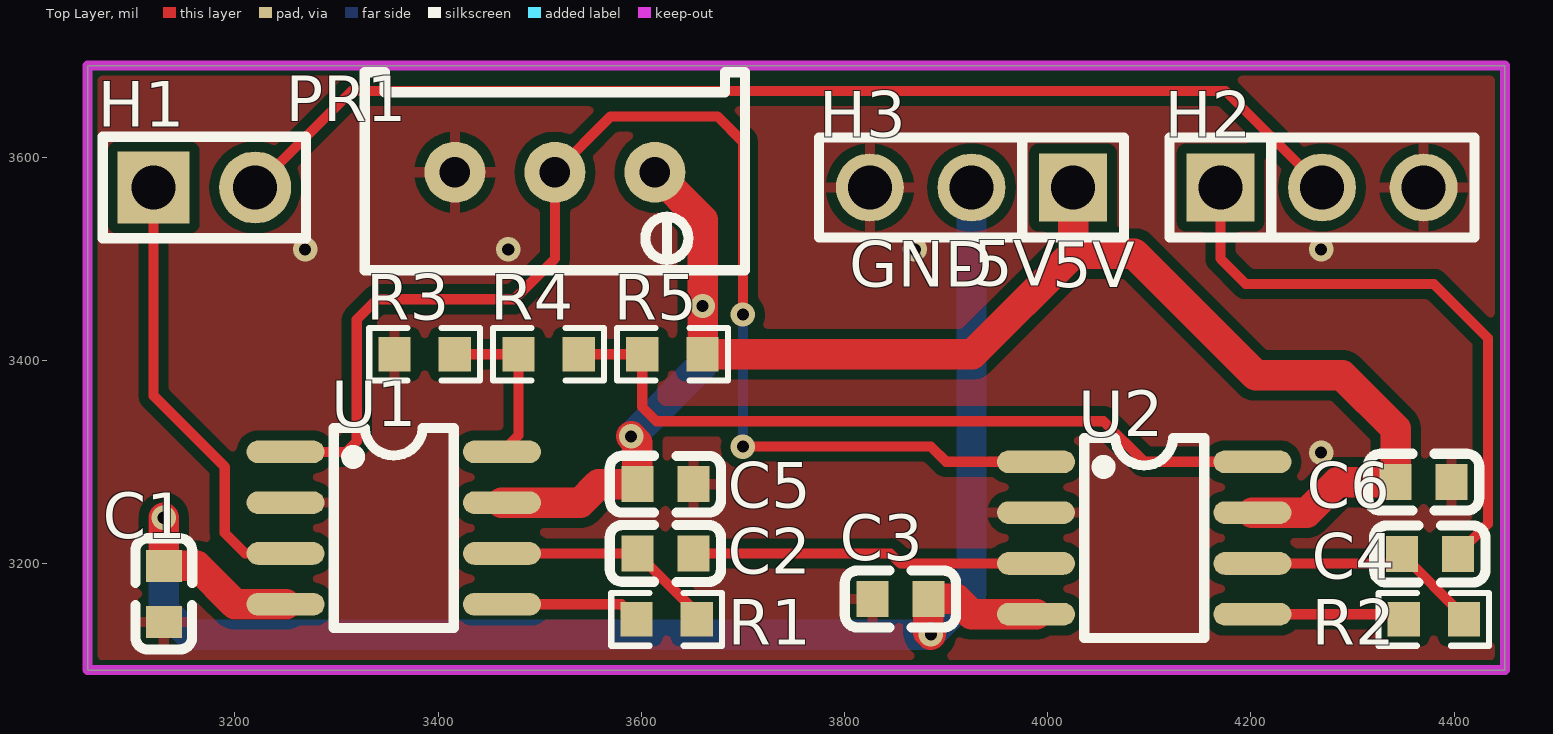
[diagram p0: Top Layer view]
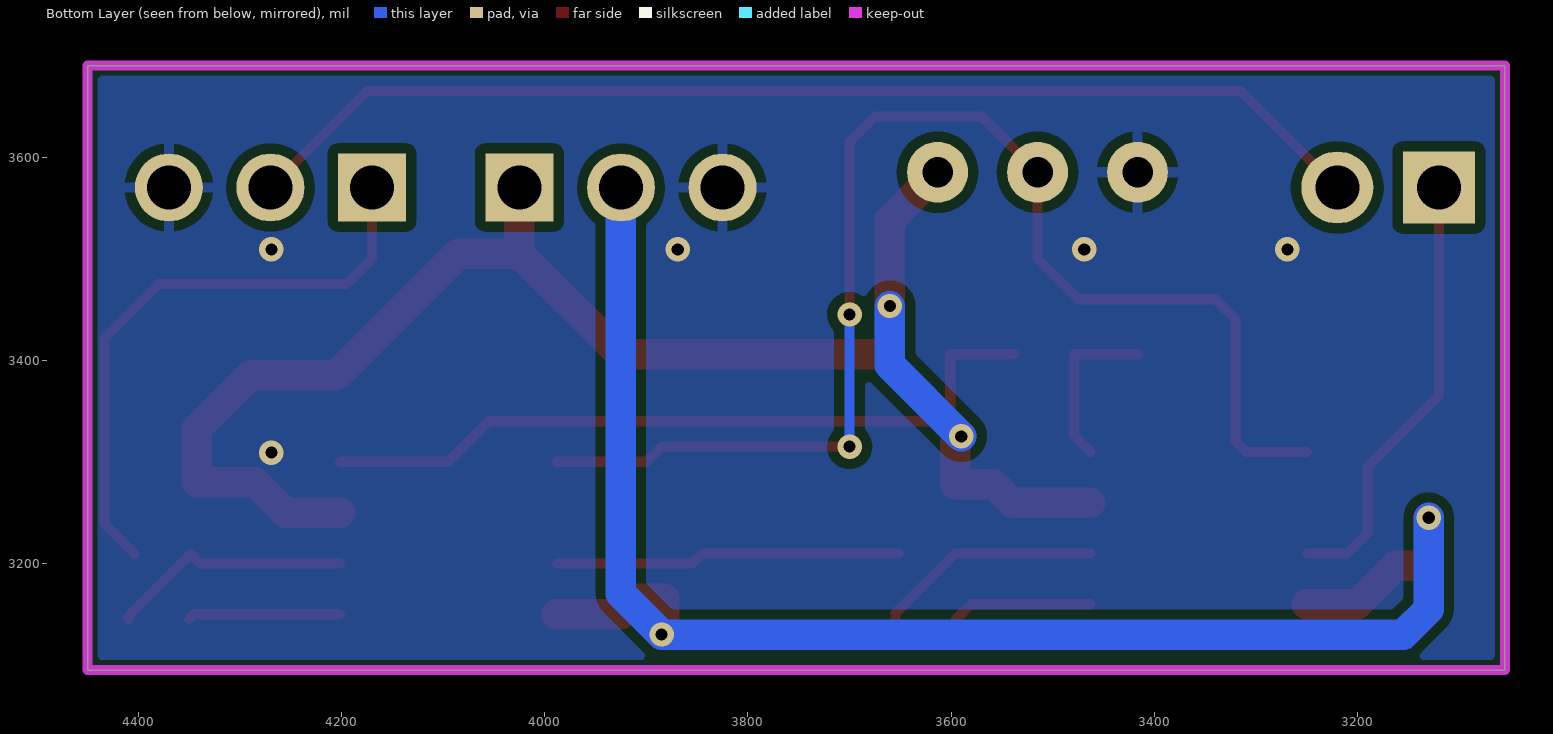
[diagram p1: Bottom Layer view, seen from below]
# Altium PCB MISC89042.pcbdoc
Units mil, origin at the board's own origin, x right, y up, seen from the top; angles counter-clockwise.
Board outline 1395 x 595 mil, 2 copper layers (Top Layer, Bottom Layer), stack 62.206 mil thick; 17 components, 14 nets, 49 pads, 11 vias.

## Layer stack, top to bottom
Top Solder Mask Layer: solder mask 0.394, Dk 3.3
Top Layer: signal copper 1.379
Dielectric1: surface 59.449, FR4, Dk 4.5
Bottom Layer: signal copper 1.378
Bottom Solder Mask Layer: solder mask 0.394, Dk 3.3

## Board outline
3055,3690 3055,3095 4450,3095 4450,3690

## Design rules (kind name [scope] priority, off if disabled: settings)
BoardOutlineClearance copperThickness2oz_1 [All] p2 off: genericclearance=7.99 ignorepadtopadclearanceinfootprint=FALSE except(0: Arc-SplitContinuation Track-SplitContinuation SMDPad-SplitContinuation THPad-SplitContinuation Via-SplitContinuation Fill-SplitContinuation Region-SplitContinuation Poly-SplitContinuation Text-SplitContinuation Hole-SplitContinuation; 5.98: Arc-CutoutEdge SMDPad-CutoutEdge THPad-CutoutEdge Via-CutoutEdge Fill-CutoutEdge Region-CutoutEdge Text-CutoutEdge; 6.93: Hole-OutlineEdge Hole-CutoutEdge; 10: Poly-OutlineEdge Poly-CutoutEdge; 11.81: Arc-OutlineEdge Track-OutlineEdge SMDPad-OutlineEdge THPad-OutlineEdge Via-OutlineEdge Fill-OutlineEdge Region-OutlineEdge Text-OutlineEdge Track-CutoutEdge)
BoardOutlineClearance copperThickness1oz_1 [All] p4: genericclearance=4.02 ignorepadtopadclearanceinfootprint=FALSE except(0: Arc-SplitContinuation Track-SplitContinuation SMDPad-SplitContinuation THPad-SplitContinuation Via-SplitContinuation Fill-SplitContinuation Region-SplitContinuation Poly-SplitContinuation Text-SplitContinuation Hole-SplitContinuation; 6: SMDPad-CutoutEdge THPad-CutoutEdge Via-CutoutEdge Fill-CutoutEdge Region-CutoutEdge Text-CutoutEdge; 6.93: Hole-OutlineEdge Hole-CutoutEdge; 10: Poly-OutlineEdge Poly-CutoutEdge; 11.8: Arc-OutlineEdge Track-OutlineEdge SMDPad-OutlineEdge THPad-OutlineEdge Via-OutlineEdge Fill-OutlineEdge Region-OutlineEdge Text-OutlineEdge; 11.81: Arc-CutoutEdge Track-CutoutEdge)
Clearance copperThickness2oz [All] p1 off: gap=7.99 ignorepadtopadclearanceinfootprint=FALSE except(5.98: SMDPad-Track SMDPad-SMDPad THPad-Track SMDPad-THPad THPad-THPad Track-Via SMDPad-Via THPad-Via Via-Via Fill-Track Region-Track Fill-SMDPad Region-SMDPad Fill-THPad Region-THPad Fill-Via Region-Via Fill-Fill Fill-Region Region-Region Arc-Track Arc-SMDPad Arc-THPad Arc-Via Fill-Arc Region-Arc Arc-Arc Text-Track SMDPad-Text Text-THPad Text-Via Fill-Text Region-Text Arc-Text Text-Text; 6.93: Hole-Track Hole-SMDPad Hole-THPad Hole-Via Fill-Hole Region-Hole Hole-Arc Hole-Text; 10: Poly-Track Poly-SMDPad Poly-THPad Poly-Via Poly-Fill Poly-Region Poly-Poly Poly-Arc Poly-Text Poly-Hole)
Clearance copperThickness1oz [All] p3: gap=4.02 ignorepadtopadclearanceinfootprint=FALSE except(5.98: SMDPad-Track SMDPad-SMDPad THPad-Track SMDPad-THPad THPad-THPad Track-Via SMDPad-Via THPad-Via Via-Via Fill-Track Region-Track Fill-SMDPad Region-SMDPad Fill-THPad Region-THPad Fill-Via Region-Via Fill-Fill Fill-Region Region-Region; 6: Arc-Track Arc-SMDPad Arc-THPad Arc-Via Fill-Arc Region-Arc Arc-Arc Text-Track SMDPad-Text Text-THPad Text-Via Fill-Text Region-Text Arc-Text Text-Text; 6.93: Hole-Track Hole-SMDPad Hole-THPad Hole-Via Fill-Hole Region-Hole Hole-Arc Hole-Text; 10: Poly-Track Poly-SMDPad Poly-THPad Poly-Via Poly-Fill Poly-Region Poly-Poly Poly-Arc Poly-Text Poly-Hole)
DiffPairsRouting differentialPair [All] p1: maxlimit=6 minlimit=6 mostfreqgap=6 toplayer_minwidth=5 toplayer_prefwidth=10 toplayer_maxwidth=100 toplayer_mingap=6 toplayer_prefgap=6 toplayer_maxgap=6 bottomlayer_minwidth=5 bottomlayer_prefwidth=10 bottomlayer_maxwidth=100 bottomlayer_mingap=6 bottomlayer_prefgap=6 bottomlayer_maxgap=6 maxuncoupledlength=10
HoleToHoleClearance otherClearance [All] p1: gap=11.81 allowstackedmicrovias=TRUE
Length netLength [All] p1: minlimit=0 maxlimit=0
MatchedLengths netLengthTolerance [All] p1: tolerance=1000
PasteMaskExpansion pasteMaskExpansion [All] p1: expansion=0
PlaneConnect innerPlane [All] p1: planeconnectstyle=Relief reliefexpansion=20 reliefentries=4 reliefconductorwidth=10 reliefairgap=10
PolygonConnect copperRegion [(InNet('GND'))] p1: connectstyle=Relief reliefconductorwidth=10 reliefentries=4 polygonreliefangle="90 Angle" airgapwidth=10 via.connectstyle=Relief via.reliefconductorwidth=10 via.reliefentries=4 via.polygonreliefangle="90 Angle" via.airgapwidth=10
RoutingVias viaSize [All] p1: holewidth=12.01 width=24.02 viastyle="Through Hole" minholewidth=11.81 minwidth=19.68 maxholewidth=248.03 maxwidth=393.7
SolderMaskExpansion solderMaskExpansion [IsVia] p1: expansion=-1000 istentingtop=TRUE
SolderMaskExpansion solderMaskExpansion [All] p2: expansion=2 istentingtop=FALSE
Width copperThickness2oz_2 [All] p1 off: maxlimit=100 minlimit=8 preferedwidth=10
Width copperThickness1oz_2 [All] p2: maxlimit=100 minlimit=5 preferedwidth=10

## Components (designator, comment, footprint, x,y, rotation, side; value= is the part's Value field where it differs from the comment)
C1 "10uF" C0603 3130,3170 r90 top
C2 "10uF" C0603 3623.7,3209.82 r0 top
C3 "10uF" C0603 3855,3165 r0 top
C4 "10uF" C0603 4376.05,3209.23 r0 top
C5 "100nF" C0603 3623.66,3277.95 r180 top
C6 "100nF" C0603 4370,3280 r180 top
H1 "" HDR-TH_2P-P2.54-V-M-1 3170,3570 r0 top
H2 "" HDR-TH_3P-P2.54-V-M 4270,3570 r0 top
H3 "" HDR-TH_3P-P2.54-V-M 3925,3570 r180 top
PR1 "1kΩ" R_3296 3515,3580 r180 top
R1 "49.4K" R0603 3625,3145 r0 top
R2 "49.4K" R0603 4380,3145 r0 top
R3 "1K" R0603 3386.76,3405.85 r0 top
R4 "1K" R0603 3508.7,3405.85 r0 top
R5 "1K" R0603 3630.63,3405.85 r0 top
U1 "AD620N" SOIC-8_L5.0-W4.0-P1.27-LS6.0-BL 3356.37,3234.82 r270 top
U2 "AD620N" SOIC-8_L5.0-W4.0-P1.27-LS6.0-BL 4095,3225 r270 top

## Footprints (in the part's own frame and the unit in brackets; to place one, negate y for a bottom-side part, rotate by r counter-clockwise, add the part's x,y. Pads: shape width x height; smd on the part's side, far side on the other; paste and mask are expansions set on the pad)
C0603 [mm]
  rect 0.8x0.9 smd: 1(-0.7,0) 2(0.7,0)
  silkscreen extent -1.39,-0.71 1.39,0.71
HDR-TH_2P-P2.54-V-M-1 [mm]
  rect 1.8x1.8 hole 1.1: 1(-1.27,0)
  round 1.8 hole 1.1: 2(1.27,0)
  silkscreen extent -2.54,-1.27 2.54,1.27
HDR-TH_3P-P2.54-V-M [mm]
  rect 1.7x1.7 hole 1.1: 1(-2.54,0)
  round 1.7 hole 1.1: 2(0,0) 3(2.54,0)
  silkscreen extent -3.81,-1.25 3.81,1.25
R0603 [mil]
  rect 31.75x34.02 smd paste-3937.01 mask+2: 1(-29.66,0) 2(29.66,0)
  silkscreen extent -55,-26 55,26
R_3296 [mil]
  round 60 hole 30 paste+0 mask+2: 1(-98.4,-5) 2(0,-5) 3(98.4,-5)
  silkscreen extent -187,-103 187,92
SOIC-8_L5.0-W4.0-P1.27-LS6.0-BL [mil]
  oval 22.38x76.78 smd: 1(-75,-106.5) 2(-25,-106.5) 3(25,-106.5) 4(75,-106.5) 5(75,106.5) 6(25,106.5) 7(-25,106.5) 8(-75,106.5)
  silkscreen extent -98,-59 98,59

## Via types
v1: diameter 24.02, hole 12, Top Layer to Bottom Layer, 11 vias

## Nets (pads, with @x,y where several pads share a name; then routed paths per layer and width w, separated by ;. In a path a pad name is that pad's centre, name@x,y a point inside that pad or via, vN(x,y) a via of type N, cw(c..) or ccw(c..) an arc to the next point about the centre after c; other vN are vias at no path point)
5V: C5.2 C6.2 H3.1 PR1.1 R5.2 U1.7 U2.7 | length 1611.9
  Top Layer w30: U1.7 3539.82,3259.82 3557.95,3277.95 C5.2 3596.1,3318.9 v1(3590,3325) ; PR1.1 3660.29,3538.11 v1(3660.29,3453.33) R5.2 3925.85,3405.85 4025,3505 ; H3.1 4025,3505 ; U2.7 4255,3250 4285,3280 C6.2 4342.44,3332.56 4290,3385 4205,3385 4085,3505 4025,3505
  Bottom Layer w30: v1(3590,3325) 3660.29,3395.29 v1(3660.29,3453.33)
$1N1: R1.1 U1.5 | length 138.6
  Top Layer w10: U1.5 3580.52,3159.82 R1.1
$1N5: H1.1 U1.3 | length 437.2
  Top Layer w10: H1.1 3120,3365 3190,3295 3190,3230 3210.18,3209.82 U1.3
$1N6: H1.2 H2.2 | length 1128.7
  Top Layer w10: H1.2 3315,3665 4175,3665 H2.2
$1N7: C2.1 R1.2 U1.6 | length 222.3
  Top Layer w10: U1.6 C2.1 3654.66,3151.3 R1.2
$1N10: C2.2 U2.3 | length 341.3
  Top Layer w10: C2.2 3845.18,3209.82 3855,3200 U2.3
$1N12: R2.1 U2.5 | length 150.9
  Top Layer w10: U2.5 4345.34,3150 R2.1
$1N13: C4.1 R2.2 U2.6 | length 240.4
  Top Layer w10: U2.6 4339.26,3200 C4.1 4409.66,3148.05 R2.2
$1N14: C4.2 H2.1 | length 590.4
  Top Layer w10: H2.1 4170,3500 4195,3475 4380,3475 4433.2,3421.8 4433.2,3238.82 C4.2
$1N16: PR1.2 U1.1 U2.1 | length 1312
  Top Layer w10: U1.1 3309.82,3309.82 3320,3320 3320,3440 3340,3460 3475,3460 3515,3500 PR1.2 3570,3640 3675,3640 3700,3615 v1(3700,3445) ; v1(3700,3315) 3885,3315 3900,3300 U2.1
  Bottom Layer w10: v1(3700,3315) v1(3700,3445)
$1N17: R3.2 R4.1 U1.8 | length 165.3
  Top Layer w10: R3.2 R4.1 3479.04,3325.99 U1.8
$1N18: R4.2 R5.1 U2.8 | length 737.3
  Top Layer w10: R4.2 R5.1 3600.97,3354.03 3615,3340 4055,3340 4095,3300 U2.8
-5V: C1.2 C3.2 H3.2 U1.4 U2.4 | length 1643
  Top Layer w30: v1(3130,3245) C1.2 3162.44,3197.56 3200.18,3159.82 U1.4 ; v1(3885,3130) 3882.56,3132.44 C3.2 3910,3165 3925,3150 U2.4
  Bottom Layer w30: v1(3130,3245) 3130,3155 3155,3130 v1(3885,3130) 3925,3170 H3.2
GND: C1.1 C3.1 C5.1 C6.1 H2.3 H3.3 PR1.3 R3.1 U1.2 U2.2
  other v1: 4269.1,3309.1 3269.1,3509.1 3469.1,3509.1 3869.1,3509.1 4269.1,3509.1

## Polygon pours and split planes (outlines as drawn)
GND on Bottom Layer (solid, remove dead copper, pour order 2): 3000,3730 3000,3040 4520,3040 4520,3730
GND on Top Layer (solid, remove dead copper, pour order 0): 3025,3750 3025,3000 4510,3000 4510,3750

## Keep-outs
Board Outline Layer:
  the board outline again, w10

## Silkscreen, mask and mechanical layers (free items; w line width, h text height)
Top Silkscreen Layer:
  text "-5V" at 3904.5,3473.46 h45
  text "GND" at 3804.5,3472.5 h45
  text "5V" at 4004.5,3471.71 h45